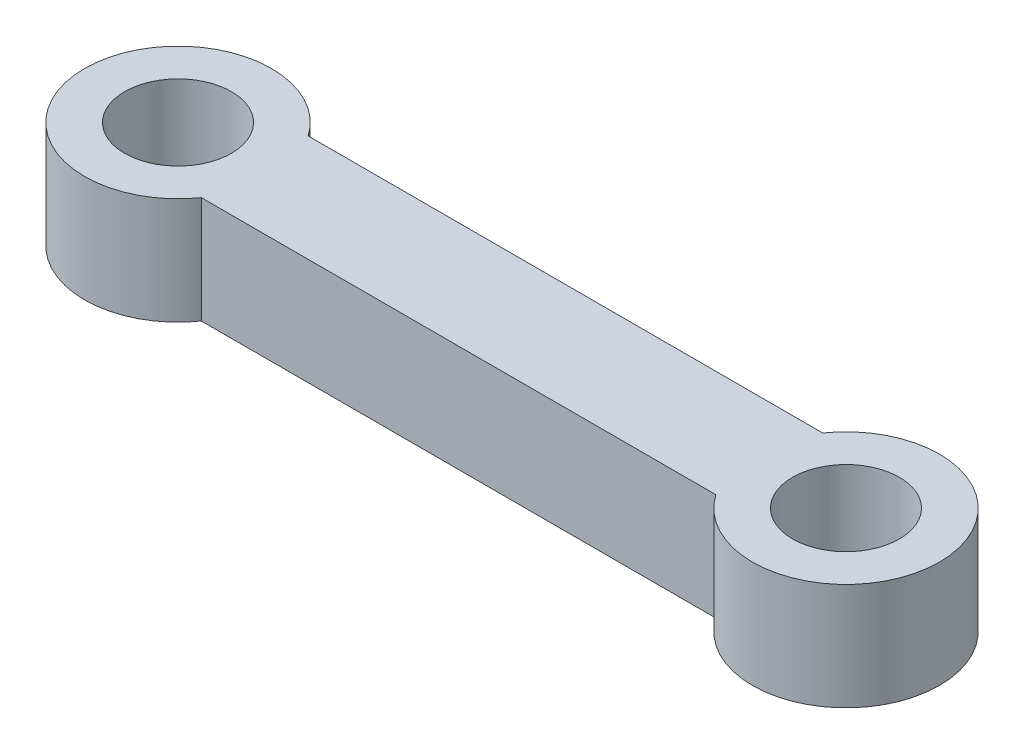
from build123d import *

# Parameters (mm, degrees)
SKETCH1_R           = 4
BOSS_EXTRUDE1_DEPTH = 8
SCALE1_SCALE        = 0.5


with BuildPart() as part:
    # Sketch1 → Boss-Extrude1 (new body)
    with BuildSketch(Plane(origin=(0, 0, 0), x_dir=(1, 0, 0), z_dir=(0, 1, 0))):
        with BuildLine():
            Line((5.744562647, 4), (44.255437353, 4))
            ThreePointArc((44.255437353, 4), (57, 0), (44.255437353, -4))
            Line((44.255437353, -4), (5.744562647, -4))
            ThreePointArc((5.744562647, -4), (-7, 0), (5.744562647, 4))
        make_face()
        with Locations(Location((0, 0, 0), (0, 0, 270))):
            Circle(SKETCH1_R, mode=Mode.SUBTRACT)
        with Locations(Location((50, 0, 0), (0, 0, 270))):
            Circle(SKETCH1_R, mode=Mode.SUBTRACT)
    extrude(amount=BOSS_EXTRUDE1_DEPTH)


with BuildPart() as part_1:
    # Scale1: scaled about (0, 0, 0)
    add(part.part.scale(SCALE1_SCALE))


solid = part_1.part
